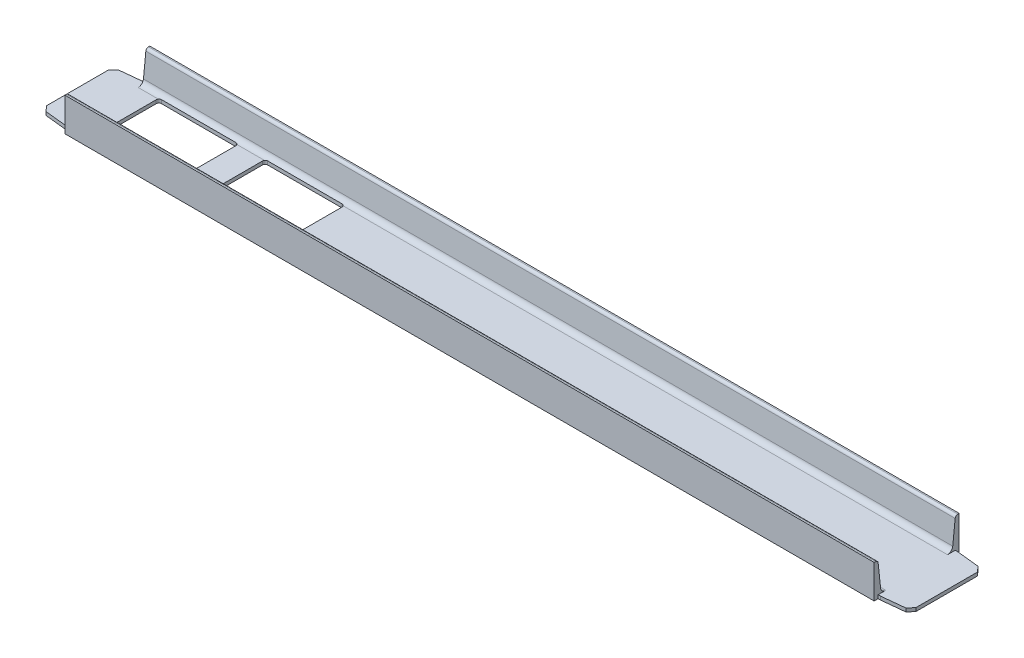
from build123d import *

# Parameters (mm, degrees)
GBT706_2008_16A_1_DEPTH = 1637
CUT_EXTRUDE_1_DEPTH     = 837.367891541
CUT_EXTRUDE_2_DEPTH     = 837.367891541
SKETCH_4_W              = 56.5
SKETCH_4_H              = 56.5
CUT_EXTRUDE_3_DEPTH     = 835.965313439
SKETCH_5_W              = 56.5
SKETCH_5_H              = 56.5
CUT_EXTRUDE_4_DEPTH     = 835.965313439
CUT_EXTRUDE_5_REACH     = 838.368


with BuildPart() as part:
    # Sketch12 → Gbt706-2008 热轧槽钢 16A(1) (new body)
    with BuildSketch(Plane.YZ.offset(-818.5)):
        with BuildLine():
            Line((63, 160), (0, 160))
            Line((0, 160), (0, 0))
            Line((0, 0), (63, 0))
            Line((63, 0), (63, 2.528785132))
            ThreePointArc((63, 2.528785132), (61.715724127, 5.874438164), (58.522642316, 7.501394609))
            Line((58.522642316, 7.501394609), (15.454715367, 12.028016136))
            ThreePointArc((15.454715367, 12.028016136), (9.068551745, 15.281929026), (6.5, 21.973235089))
            Line((6.5, 21.973235089), (6.5, 138.026764911))
            ThreePointArc((6.5, 138.026764911), (9.068551745, 144.718070974), (15.454715367, 147.971983864))
            Line((15.454715367, 147.971983864), (58.522642316, 152.498605391))
            ThreePointArc((58.522642316, 152.498605391), (61.715724127, 154.125561836), (63, 157.471214868))
            Line((63, 157.471214868), (63, 160))
        make_face()
    extrude(amount=GBT706_2008_16A_1_DEPTH)

    # 草图2 → 切除-拉伸1 (cut, through all)
    with BuildSketch(Plane.XZ):
        Polygon((762, -5), (762, 7.501394609), (766.477357684, 7.501394609), (809.545284633, 12.028016136), (818.5, 21.973235089), (818.5, 138.026764911), (809.545284633, 147.971983864), (766.477357684, 152.498605391), (762, 152.498605391), (762, 165), (828.5, 165), (828.5, -5), align=None)
    extrude(amount=-CUT_EXTRUDE_1_DEPTH, mode=Mode.SUBTRACT)

    # 草图3 → 切除-拉伸2 (cut, through all)
    with BuildSketch(Plane.XZ):
        Polygon((-762, 0), (-762, 7.501394609), (-766.477357684, 7.501394609), (-809.545284633, 12.028016136), (-818.5, 21.973235089), (-818.5, 138.026764911), (-809.545284633, 147.971983864), (-766.477357684, 152.498605391), (-762, 152.498605391), (-762, 165), (-838.5, 165), (-838.5, -5), (-762, -5), align=None)
    extrude(amount=-CUT_EXTRUDE_2_DEPTH, mode=Mode.SUBTRACT)

    # 草图4 → 切除-拉伸3 (cut, through all)
    with BuildSketch(Plane.XY.offset(152.498605391)):
        with Locations((790.25, 34.75)):
            Rectangle(SKETCH_4_W, SKETCH_4_H)
    extrude(amount=-CUT_EXTRUDE_3_DEPTH, mode=Mode.SUBTRACT)

    # 草图5 → 切除-拉伸4 (cut, through all)
    with BuildSketch(Plane.XY.offset(152.498605391)):
        with Locations((-790.25, 34.75)):
            Rectangle(SKETCH_5_W, SKETCH_5_H)
    extrude(amount=-CUT_EXTRUDE_4_DEPTH, mode=Mode.SUBTRACT)

    # 草图6 → 切除-拉伸5 (cut, up to next)
    with BuildSketch(Plane.XZ, mode=Mode.PRIVATE) as cut_extrude_5_sk1:
        with BuildLine():
            Line((-580, 20), (-720, 20))
            ThreePointArc((-720, 20), (-723.535533906, 21.464466094), (-725, 25))
            Line((-725, 25), (-725, 105))
            ThreePointArc((-725, 105), (-723.535533906, 108.535533906), (-720, 110))
            Line((-720, 110), (-580, 110))
            ThreePointArc((-580, 110), (-576.464466094, 108.535533906), (-575, 105))
            Line((-575, 105), (-575, 25))
            ThreePointArc((-575, 25), (-576.464466094, 21.464466094), (-580, 20))
        make_face()
    cut_extrude_5_tool1 = extrude(cut_extrude_5_sk1.sketch, amount=-CUT_EXTRUDE_5_REACH, mode=Mode.PRIVATE) & part.part
    # 草图6 → 切除-拉伸5 (cut, up to next)
    with BuildSketch(Plane.XZ, mode=Mode.PRIVATE) as cut_extrude_5_sk2:
        with BuildLine():
            Line((-375, 25), (-375, 105))
            ThreePointArc((-375, 105), (-376.464466094, 108.535533906), (-380, 110))
            Line((-380, 110), (-520, 110))
            ThreePointArc((-520, 110), (-523.535533906, 108.535533906), (-525, 105))
            Line((-525, 105), (-525, 25))
            ThreePointArc((-525, 25), (-523.535533906, 21.464466094), (-520, 20))
            Line((-520, 20), (-380, 20))
            ThreePointArc((-380, 20), (-376.464466094, 21.464466094), (-375, 25))
        make_face()
    cut_extrude_5_tool2 = extrude(cut_extrude_5_sk2.sketch, amount=-CUT_EXTRUDE_5_REACH, mode=Mode.PRIVATE) & part.part
    add(cut_extrude_5_tool1.solids().sort_by_distance((-650, 0, 65))[0], mode=Mode.SUBTRACT)
    add(cut_extrude_5_tool2.solids().sort_by_distance((-450, 0, 65))[0], mode=Mode.SUBTRACT)


solid = part.part
